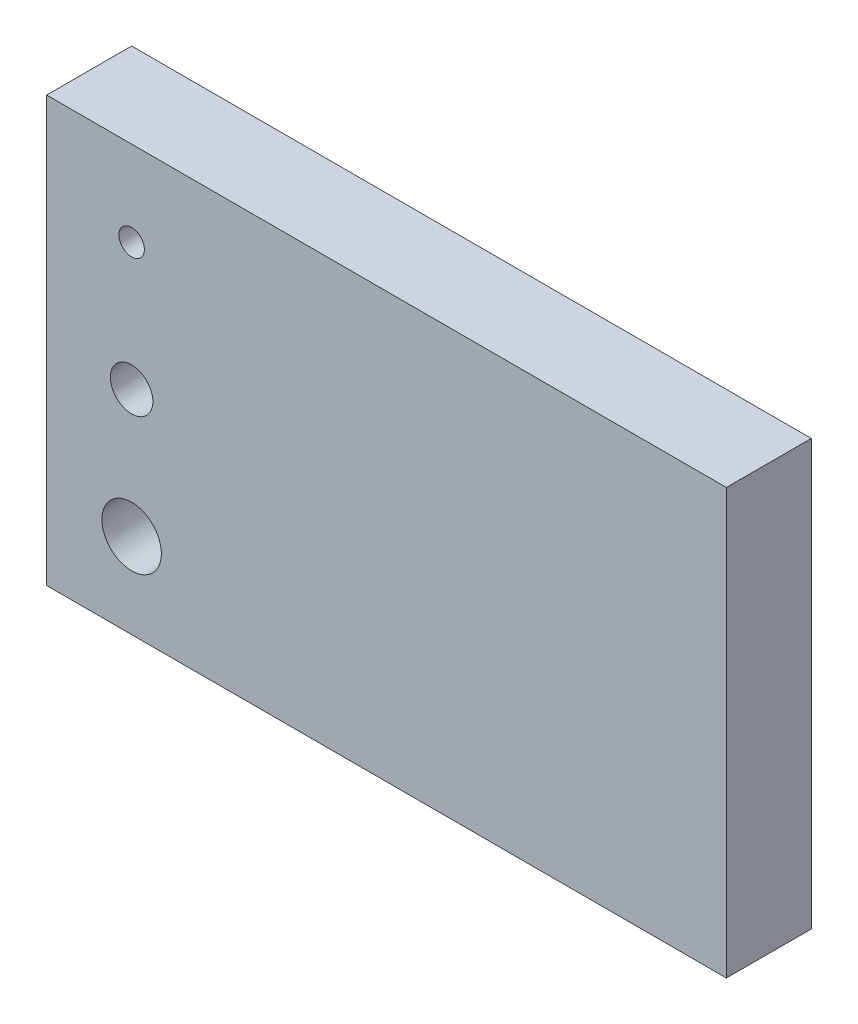
SolidWorks part; units mm, degrees
ref_plane "Front Plane" through (0, 0, 0) normal (0, 0, 1) x (1, 0, 0)
ref_plane "Top Plane" through (0, 0, 0) normal (0, 1, 0) x (1, 0, 0)
ref_plane "Right Plane" through (0, 0, 0) normal (1, 0, 0) x (0, 0, -1)
sketch "Sketch1" plane through (0, 0, 0) normal (0, 0, 1) x (1, 0, 0)
  line L1 (0, 0) -> (8, 0)
  line L2 (0, 0) -> (0, -6)
  line L3 (0, -6) -> (8, -6)
  line L4 (8, 0) -> (8, -6)
extrude "Boss-Extrude1" add sketch "Sketch1" along normal blind 1
sketch "Sketch2" plane through (0, 0, 1) normal (0, 0, 1) x (1, 0, 0)
  line L0 (0, 0) -> (0, -6) construction
  line L1 (8, 0) -> (0, 0) construction
  circle A0 centre (1, -1.5) radius 0.15
  circle A1 centre (1, -3) radius 0.25
  circle A2 centre (1, -4.5) radius 0.35
  dimension "D1" = 1
  dimension "D2" = 1.5
  dimension "D3" = 1.5
  dimension "D4" = 1.5
extrude "Cut-Extrude1" cut sketch "Sketch2" against normal blind 2
sketch "Sketch3" plane through (0, 0, 1) normal (0, 0, 1) x (1, 0, 0)
  line L0 (8, -6) -> (8, 0) construction
  line L1 (0, 0) -> (8, 0)
  line L2 (0, 0) -> (0, -0.5)
  line L3 (0, -0.5) -> (8, -0.5)
  line L4 (8, 0) -> (8, -0.5)
  line L6 (0, -6) -> (8, -6)
  line L7 (0, -6) -> (0, -5.5)
  line L8 (0, -5.5) -> (8, -5.5)
  line L9 (8, -6) -> (8, -5.5)
extrude "Cut-Extrude2" cut sketch "Sketch3" against normal blind 7
